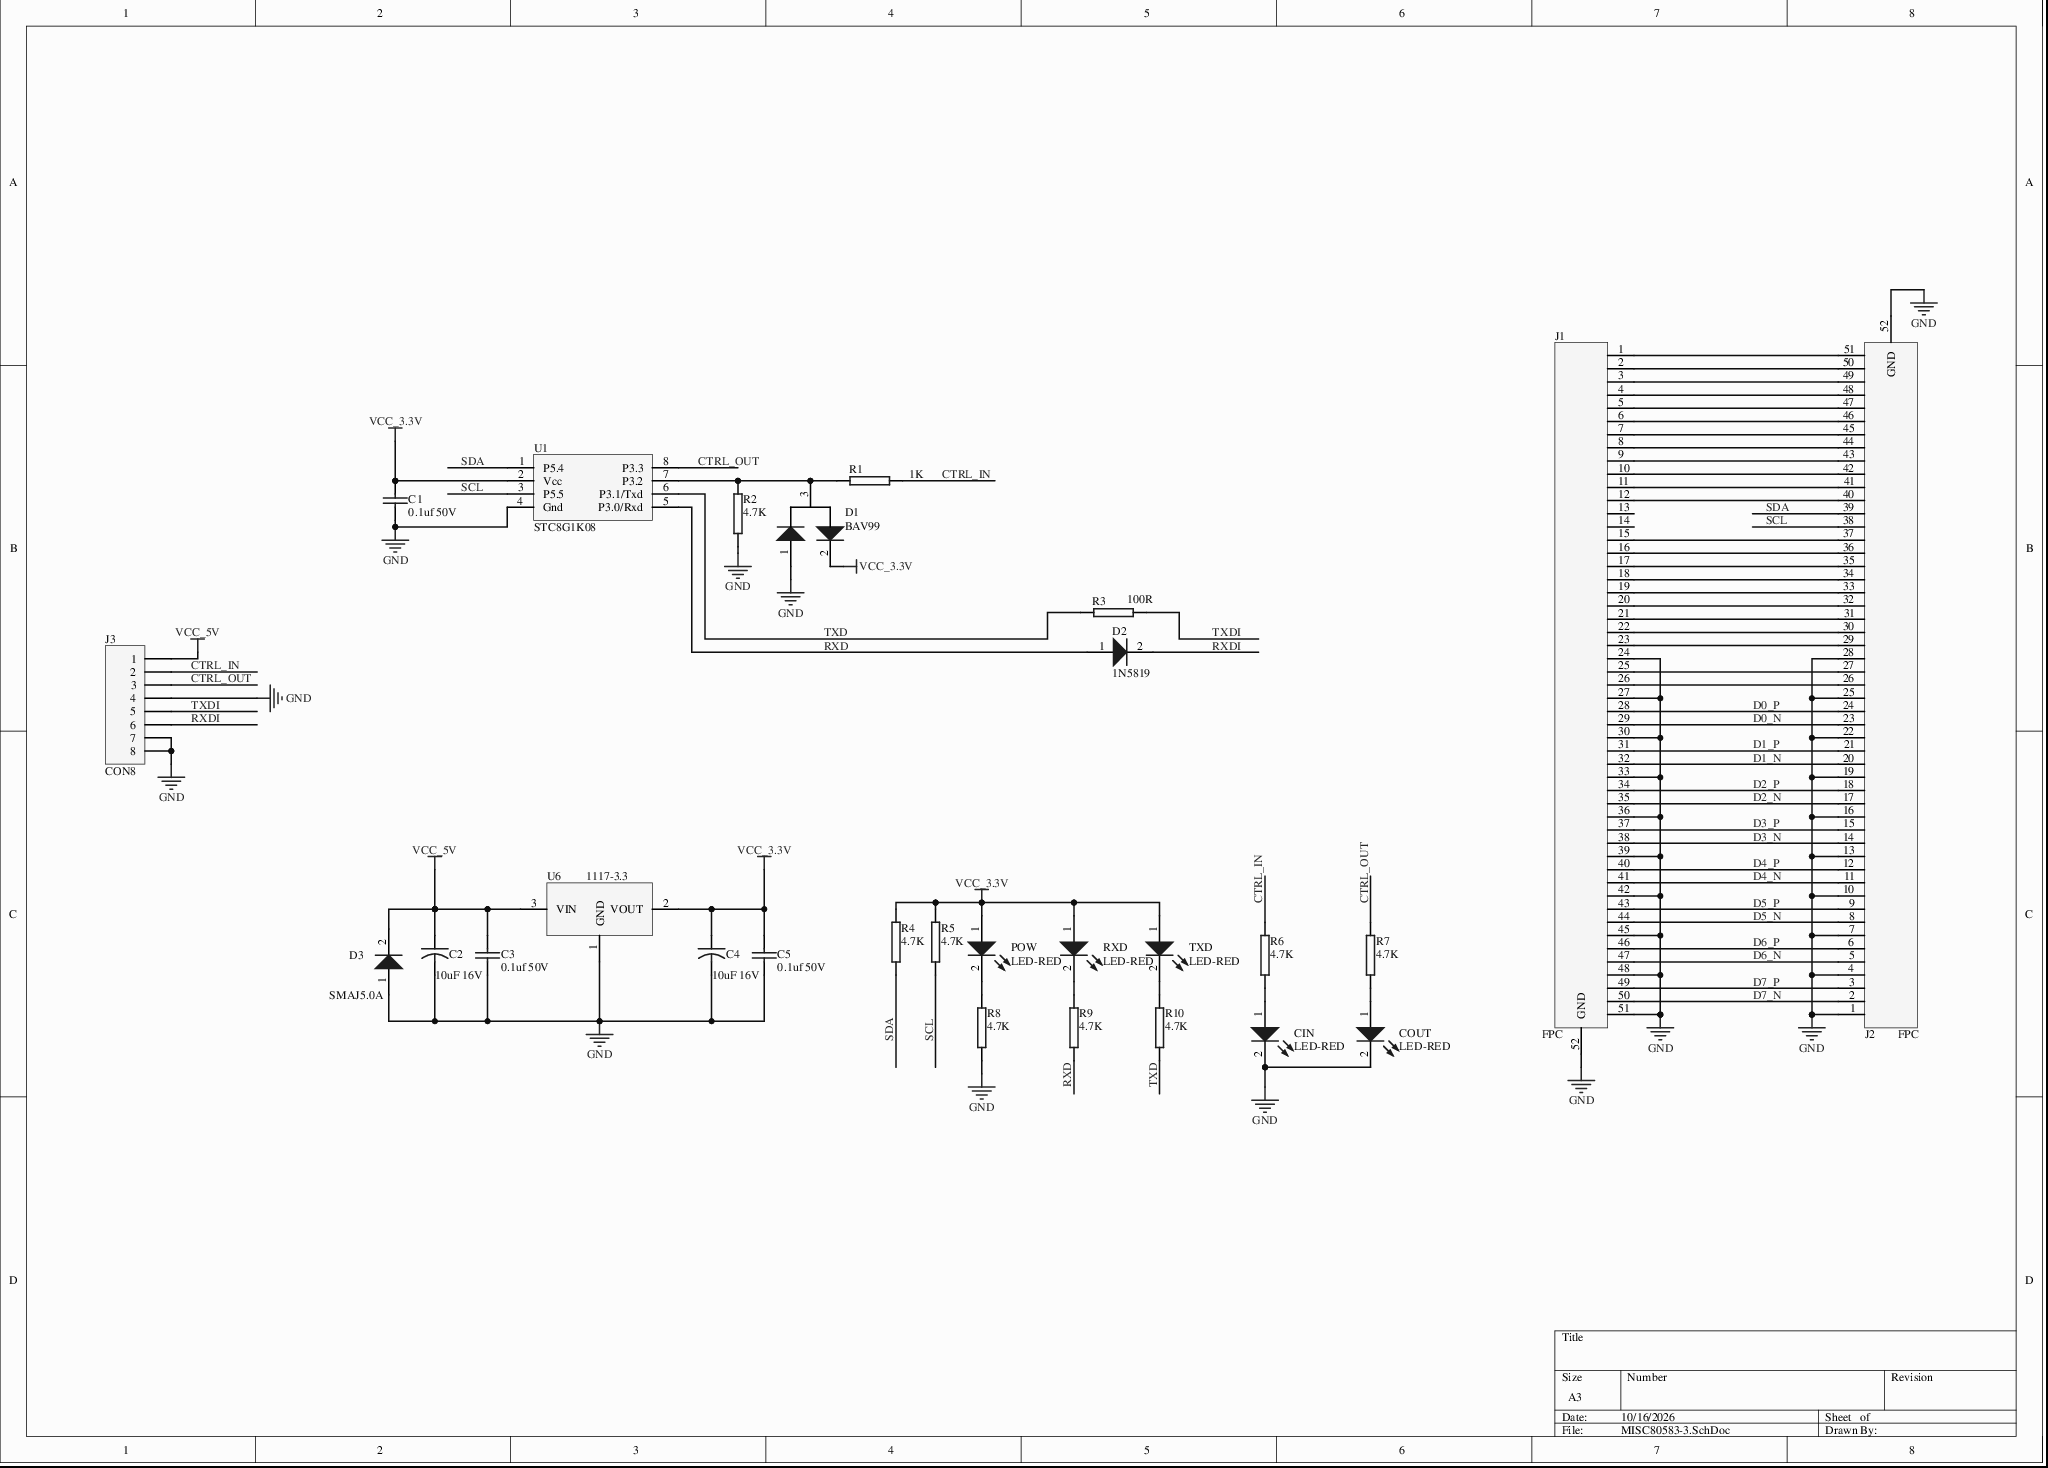
[diagram p0: MISC80583-3.SchDoc]
# Altium project MISC80583-2.PrjPcb
1 sheet, 28 parts. Net scope: global (net labels, ports and power ports of the same name join across sheets).
Board file: MISC80583.PcbDoc

## Sheet MISC80583-3.SchDoc
size A3

### Parts
C1  0.1uf 50V  [0603C]
C2  10uF 16V  [0805C]
C3  0.1uf 50V  [0603C]
C4  10uF 16V  [0805C]
C5  0.1uf 50V  [0603C]
CIN  LED-RED  [LED0603]
COUT  LED-RED  [LED0603]
D1  BAV99  [SOT-23]
D2  1N5819  [SOD-323]
D3  SMAJ5.0A  [1N5822]
J1  FPC  [FPC-0.5-51P]
J2  FPC  [FPC-0.5-51P]
J3  CON8  [CON6-Lay]
POW  LED-RED  [LED0603]
R1  1K  [0603R]
R2  4.7K  [0603R]
R3  100R  [0603R]
R4  4.7K  [0603R]
R5  4.7K  [0603R]
R6  4.7K  [0603R]
R7  4.7K  [0603R]
R8  4.7K  [0603R]
R9  4.7K  [0603R]
R10  4.7K  [0603R]
RXD  LED-RED  [LED0603]
TXD  LED-RED  [LED0603]
U1  STC8G1K08  [so-8]
U6  1117-3.3  [SOT-223]

### Nets
GND: C1.1 C2.2 C3.2 C4.2 C5.2 CIN.2(K) COUT.2(K) D1.1(A) D3.1(A) J1.24 J1.27 J1.30 J1.33 J1.36 J1.39 J1.42 J1.45 J1.48 J1.51 J1.52(GND) J2.1 J2.4 J2.7 J2.10 J2.13 J2.16 J2.19 J2.22 J2.25 J2.28 J2.52(GND) J3.4 J3.7 J3.8 R2.1 R8.1 U1.4(Gnd) U6.1(GND)
VCC_3.3V: C1.2 C4.1 C5.1 D1.2(K) POW.1(A) R4.2 R5.2 RXD.1(A) TXD.1(A) U1.2(Vcc) U6.2(VOUT)
VCC_5V: C2.1 C3.1 D3.2(K) J3.1 U6.3(VIN)
CTRL_IN: J3.2 R1.2 R6.2
CTRL_OUT: J3.3 R7.2 U1.8(P3.3)
D0_N: J1.29 J2.23
D0_P: J1.28 J2.24
D1_N: J1.32 J2.20
D1_P: J1.31 J2.21
D2_N: J1.35 J2.17
D2_P: J1.34 J2.18
D3_N: J1.38 J2.14
D3_P: J1.37 J2.15
D4_N: J1.41 J2.11
D4_P: J1.40 J2.12
D5_N: J1.44 J2.8
D5_P: J1.43 J2.9
D6_N: J1.47 J2.5
D6_P: J1.46 J2.6
D7_N: J1.50 J2.2
D7_P: J1.49 J2.3
RXD: D2.1(A) R9.1 U1.5(P3.0/Rxd)
RXDI: D2.2(K) J3.6
SCL: J2.38 R5.1 U1.3(P5.5)
SDA: J2.39 R4.1 U1.1(P5.4)
TXD: R3.1 R10.1 U1.6(P3.1/Txd)
TXDI: J3.5 R3.2
NetCIN_1: CIN.1(A) R6.1
NetCOUT_1: COUT.1(A) R7.1
NetD1_3: D1.3(K) R1.1 R2.2 U1.7(P3.2)
NetJ1_1: J1.1 J2.51
NetJ1_2: J1.2 J2.50
NetJ1_3: J1.3 J2.49
NetJ1_4: J1.4 J2.48
NetJ1_5: J1.5 J2.47
NetJ1_6: J1.6 J2.46
NetJ1_7: J1.7 J2.45
NetJ1_8: J1.8 J2.44
NetJ1_9: J1.9 J2.43
NetJ1_10: J1.10 J2.42
NetJ1_11: J1.11 J2.41
NetJ1_12: J1.12 J2.40
NetJ1_15: J1.15 J2.37
NetJ1_16: J1.16 J2.36
NetJ1_17: J1.17 J2.35
NetJ1_18: J1.18 J2.34
NetJ1_19: J1.19 J2.33
NetJ1_20: J1.20 J2.32
NetJ1_21: J1.21 J2.31
NetJ1_22: J1.22 J2.30
NetJ1_23: J1.23 J2.29
NetJ1_25: J1.25 J2.27
NetJ1_26: J1.26 J2.26
NetPOW_2: POW.2(K) R8.2
NetR9_2: R9.2 RXD.2(K)
NetR10_2: R10.2 TXD.2(K)

Not connected (* = marked no-connect by the designer): J1 13(12) 14(13)

### Layout directives
differential pair: D0_N, D0_P, D1_N, D1_P, D2_N, D2_P, D3_N, D3_P, D4_N, D4_P, D5_N, D5_P, D6_N, D6_P, D7_N, D7_P

### Library data of the parts
C1 C3 C5 = CAP: Capacitor
C2 C4 = CAPACITOR
CIN COUT POW RXD TXD = LED2: Typical RED, GREEN, YELLOW, AMBER GaAs LED; Published: 8-Jun-2000; Revision: July-2002: Re-released for DXP Platform.; Publisher: Altium Limited
D3 = 1N5819
J1 J2 = FPC-0.5-51P
J3 = CON8: Connector
R1-R10 = RES2
U6 = AS1117